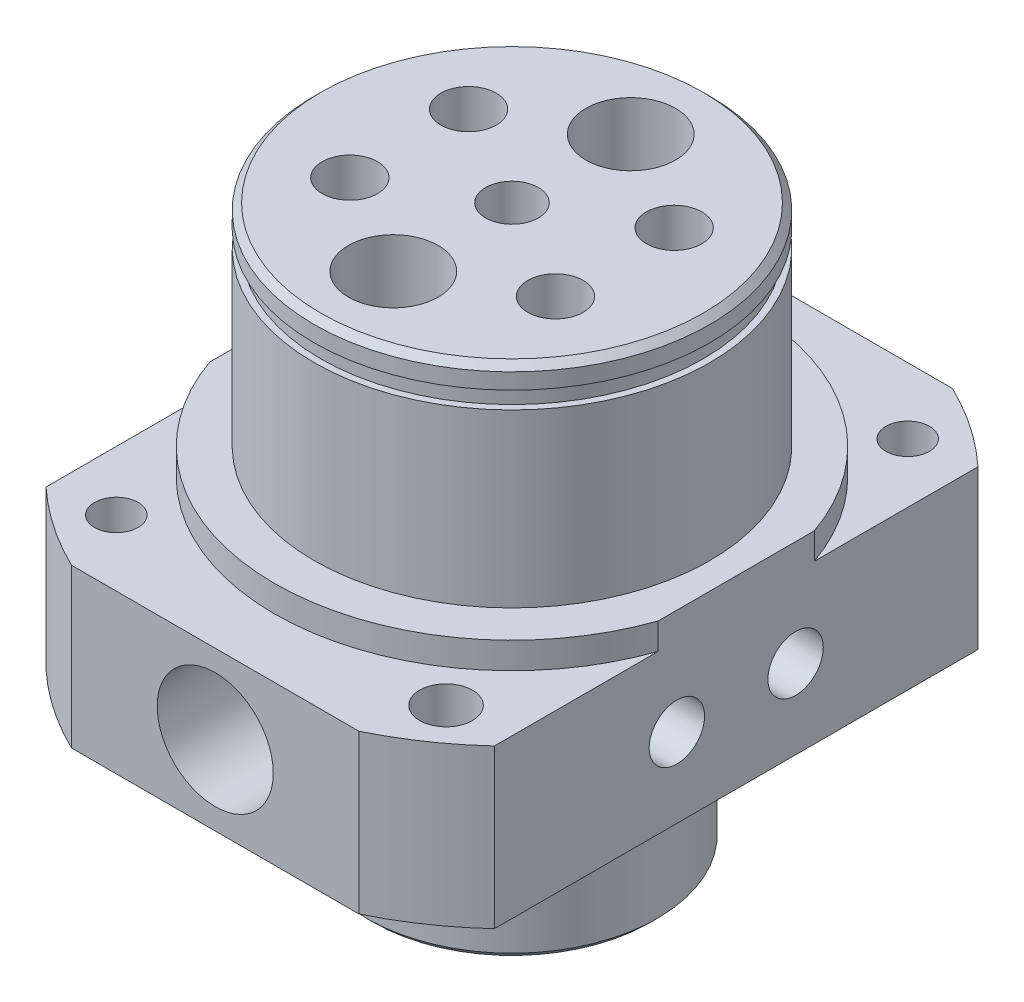
from build123d import *

# Parameters (mm, degrees)
SKETCH2_OUTSIDE_W        = 68.448
SKETCH2_OUTSIDE_H        = 68.448
SKETCH2_OUTSIDE_W_2      = 34
SKETCH2_OUTSIDE_H_2      = 45
CUT_EXTRUDE1_DEPTH       = 47.368092477
M4_TAPPED_HOLE1_D        = 3.3
SKETCH14_R               = 2
CUT_EXTRUDE5_DEPTH       = 38.030392923
SKETCH17_R               = 2
SKETCH17_R_2             = 3
CUT_EXTRUDE7_DEPTH       = 28
CUT_EXTRUDE10_REACH      = 52.619
SKETCH18_R               = 2
CUT_EXTRUDE11_REACH      = 52.619
SKETCH19_R               = 2
CUT_EXTRUDE12_REACH      = 58.692
CUT_EXTRUDE12_END_RADIUS = 3
SKETCH20_R               = 3
CUT_EXTRUDE13_REACH      = 58.692
CUT_EXTRUDE13_END_RADIUS = 3
SKETCH21_R               = 3
SKETCH22_R               = 2
CUT_EXTRUDE14_DEPTH      = 51.589030432
CHAMFER1_SIZE            = 0.5
M8_TAPPED_HOLE1_D        = 6.8
M8_TAPPED_HOLE1_DEPTH    = 15
M8_TAPPED_HOLE1_TIP      = 2.042926105
M5_TAPPED_HOLE2_D        = 4.2
M5_TAPPED_HOLE2_DEPTH    = 12
M5_TAPPED_HOLE2_TIP      = 1.2618073
M5_TAPPED_HOLE1_D        = 4.2
M5_TAPPED_HOLE1_DEPTH    = 12
M5_TAPPED_HOLE1_TIP      = 1.2618073
M5_TAPPED_HOLE3_D        = 4.2
M5_TAPPED_HOLE3_DEPTH    = 12
M5_TAPPED_HOLE3_TIP      = 1.2618073
G1_8_TAPPED_HOLE1_D      = 8.8
G1_8_TAPPED_HOLE1_DEPTH  = 15
G1_8_TAPPED_HOLE1_TIP    = 2.643786724
G1_8_TAPPED_HOLE2_D      = 8.8
G1_8_TAPPED_HOLE2_DEPTH  = 15
G1_8_TAPPED_HOLE2_TIP    = 2.643786724


with BuildPart() as part:
    # Sketch1 → Revolve1 (revolve)
    with BuildSketch(Plane(origin=(0, 0, 0), x_dir=(0, 0, -1), z_dir=(1, 0, 0)), mode=Mode.PRIVATE) as revolve1_sk:
        Polygon((0, -12), (11, -12), (11, 0), (25, 0), (25, 12), (18, 12), (18, 14), (15, 14), (15, 27), (14.5, 27), (14.5, 28.3), (15, 28.3), (15, 30), (0, 30), align=None)
    revolve(revolve1_sk.sketch.rotate(Axis((0, 78.762169225, 0), (0, -1, 0)), 180), axis=Axis((0, 78.762169225, 0), (0, -1, 0)))

    # Sketch2 outside → Cut-Extrude1 (cut, through all)
    with BuildSketch(Plane(origin=(0, 0, 0), x_dir=(1, 0, 0), z_dir=(0, 1, 0))):
        Rectangle(SKETCH2_OUTSIDE_W, SKETCH2_OUTSIDE_H)
        Rectangle(SKETCH2_OUTSIDE_W_2, SKETCH2_OUTSIDE_H_2, mode=Mode.SUBTRACT)
    extrude(amount=CUT_EXTRUDE1_DEPTH, mode=Mode.SUBTRACT)

    # M4 Tapped Hole1 (through all)
    with Locations(Plane(origin=(0, 0, 0), x_dir=(-1, 0, 0), z_dir=(0, -1, 0))):
        with Locations((-12.5, 17.5), (12.5, -17.5)):
            Hole(M4_TAPPED_HOLE1_D / 2)

    # Sketch14 → Cut-Extrude5 (cut, through all)
    with BuildSketch(Plane(origin=(0, 12, 0), x_dir=(1, 0, 0), z_dir=(0, 1, 0))):
        with Locations(Location((12.5, -17.5, 0), (0, 0, 270))):
            Circle(SKETCH14_R)
        with Locations(Location((-12.5, 17.5, 0), (0, 0, 270))):
            Circle(SKETCH14_R)
    extrude(amount=-CUT_EXTRUDE5_DEPTH, mode=Mode.SUBTRACT)

    # Sketch17 → Cut-Extrude7 (cut)
    with BuildSketch(Plane(origin=(0, 30, 0), x_dir=(1, 0, 0), z_dir=(0, 1, 0))):
        with Locations(Location((-7.794228634, 4.5, 0), (0, 0, 270))):
            Circle(SKETCH17_R)
        with Locations(Location((-7.794228634, -4.5, 0), (0, 0, 270))):
            Circle(SKETCH17_R)
        with Locations(Location((0, -9, 0), (0, 0, 270))):
            Circle(SKETCH17_R_2)
        with Locations(Location((7.794228634, 4.5, 0), (0, 0, 270))):
            Circle(SKETCH17_R)
        with Locations(Location((0, 9, 0), (0, 0, 270))):
            Circle(SKETCH17_R_2)
        with Locations(Location((7.794228634, -4.5, 0), (0, 0, 270))):
            Circle(SKETCH17_R)
        with Locations(Location((0, 0, 0), (0, 0, 270))):
            Circle(SKETCH17_R)
    extrude(amount=-CUT_EXTRUDE7_DEPTH, mode=Mode.SUBTRACT)

    # Sketch18 → Cut-Extrude10 (cut, up to next)
    with BuildSketch(Plane.ZY.offset(17), mode=Mode.PRIVATE) as cut_extrude10_sk1:
        with Locations((-4.5, 6)):
            Circle(SKETCH18_R)
    cut_extrude10_tool1 = extrude(cut_extrude10_sk1.sketch, amount=-CUT_EXTRUDE10_REACH, mode=Mode.PRIVATE) & part.part
    # Sketch18 → Cut-Extrude10 (cut, up to next)
    with BuildSketch(Plane.ZY.offset(17), mode=Mode.PRIVATE) as cut_extrude10_sk2:
        with Locations((4.5, 6)):
            Circle(SKETCH18_R)
    cut_extrude10_tool2 = extrude(cut_extrude10_sk2.sketch, amount=-CUT_EXTRUDE10_REACH, mode=Mode.PRIVATE) & part.part
    add(cut_extrude10_tool1.solids().sort_by_distance((-17, 6, -4.5))[0], mode=Mode.SUBTRACT)
    add(cut_extrude10_tool2.solids().sort_by_distance((-17, 6, 4.5))[0], mode=Mode.SUBTRACT)

    # Sketch19 → Cut-Extrude11 (cut, up to next)
    with BuildSketch(Plane(origin=(17, 0, 0), x_dir=(0, 0, -1), z_dir=(1, 0, 0)), mode=Mode.PRIVATE) as cut_extrude11_sk1:
        with Locations(Location((-4.5, 6, 0), (0, 0, 180))):
            Circle(SKETCH19_R)
    cut_extrude11_tool1 = extrude(cut_extrude11_sk1.sketch, amount=-CUT_EXTRUDE11_REACH, mode=Mode.PRIVATE) & part.part
    # Sketch19 → Cut-Extrude11 (cut, up to next)
    with BuildSketch(Plane(origin=(17, 0, 0), x_dir=(0, 0, -1), z_dir=(1, 0, 0)), mode=Mode.PRIVATE) as cut_extrude11_sk2:
        with Locations(Location((4.5, 6, 0), (0, 0, 180))):
            Circle(SKETCH19_R)
    cut_extrude11_tool2 = extrude(cut_extrude11_sk2.sketch, amount=-CUT_EXTRUDE11_REACH, mode=Mode.PRIVATE) & part.part
    add(cut_extrude11_tool1.solids().sort_by_distance((17, 6, 4.5))[0], mode=Mode.SUBTRACT)
    add(cut_extrude11_tool2.solids().sort_by_distance((17, 6, -4.5))[0], mode=Mode.SUBTRACT)

    # Cut-Extrude12: up to this cylinder (the profile starts outside it)
    cut_extrude12_end = Plane(origin=(0, 6, -9), z_dir=(0, 1, 0)) * Cylinder(CUT_EXTRUDE12_END_RADIUS, 124.384, mode=Mode.PRIVATE)
    # Sketch20 → Cut-Extrude12 (cut, up to the surface)
    with BuildSketch(Plane(origin=(0, 0, -22.5), x_dir=(-1, 0, 0), z_dir=(0, 0, -1)), mode=Mode.PRIVATE) as cut_extrude12_sk1:
        with Locations((0, 6)):
            Circle(SKETCH20_R)
    cut_extrude12_tool1 = extrude(cut_extrude12_sk1.sketch, amount=-CUT_EXTRUDE12_REACH, mode=Mode.PRIVATE) - cut_extrude12_end
    add(cut_extrude12_tool1.solids().sort_by_distance((0, 6, -22.5))[0], mode=Mode.SUBTRACT)

    # Cut-Extrude13: up to this cylinder (the profile starts outside it)
    cut_extrude13_end = Plane(origin=(0, 6, 9), z_dir=(0, 1, 0)) * Cylinder(CUT_EXTRUDE13_END_RADIUS, 124.384, mode=Mode.PRIVATE)
    # Sketch21 → Cut-Extrude13 (cut, up to the surface)
    with BuildSketch(Plane.XY.offset(22.5), mode=Mode.PRIVATE) as cut_extrude13_sk1:
        with Locations(Location((0, 6, 0), (0, 0, 180))):
            Circle(SKETCH21_R)
    cut_extrude13_tool1 = extrude(cut_extrude13_sk1.sketch, amount=-CUT_EXTRUDE13_REACH, mode=Mode.PRIVATE) - cut_extrude13_end
    add(cut_extrude13_tool1.solids().sort_by_distance((0, 6, 22.5))[0], mode=Mode.SUBTRACT)

    # Sketch22 → Cut-Extrude14 (cut, through all)
    with BuildSketch(Plane.XZ.offset(12)):
        with Locations(Location((0, 0, 0), (0, 0, 90))):
            Circle(SKETCH22_R)
    extrude(amount=-CUT_EXTRUDE14_DEPTH, mode=Mode.SUBTRACT)

    # Chamfer1
    chamfer1_edges = [part.edges().sort_by_distance(p)[0] for p in [
        (0, -12, -11),
        (0, 30, -15),
    ]]
    chamfer(chamfer1_edges, length=CHAMFER1_SIZE)

    # M8 Tapped Hole1
    with Locations(Plane(origin=(0, 30, 0), x_dir=(1, 0, 0), z_dir=(0, 1, 0))):
        with Locations((0, 9), (0, -9)):
            Hole(M8_TAPPED_HOLE1_D / 2, depth=M8_TAPPED_HOLE1_DEPTH)
            with Locations((0, 0, -(M8_TAPPED_HOLE1_DEPTH + M8_TAPPED_HOLE1_TIP / 2))):  # 118° drill point
                Cone(0, M8_TAPPED_HOLE1_D / 2, M8_TAPPED_HOLE1_TIP, mode=Mode.SUBTRACT)

    # M5 Tapped Hole2
    with Locations(Plane(origin=(0, 30, 0), x_dir=(1, 0, 0), z_dir=(0, 1, 0))):
        with Locations((7.794228634, 4.5), (7.794228634, -4.5), (-7.794228634, -4.5), (-7.794228634, 4.5)):
            Hole(M5_TAPPED_HOLE2_D / 2, depth=M5_TAPPED_HOLE2_DEPTH)
            with Locations((0, 0, -(M5_TAPPED_HOLE2_DEPTH + M5_TAPPED_HOLE2_TIP / 2))):  # 118° drill point
                Cone(0, M5_TAPPED_HOLE2_D / 2, M5_TAPPED_HOLE2_TIP, mode=Mode.SUBTRACT)

    # M5 Tapped Hole1
    with Locations(Plane.ZY.offset(17)):
        with Locations((-4.5, 6), (4.5, 6)):
            Hole(M5_TAPPED_HOLE1_D / 2, depth=M5_TAPPED_HOLE1_DEPTH)
            with Locations((0, 0, -(M5_TAPPED_HOLE1_DEPTH + M5_TAPPED_HOLE1_TIP / 2))):  # 118° drill point
                Cone(0, M5_TAPPED_HOLE1_D / 2, M5_TAPPED_HOLE1_TIP, mode=Mode.SUBTRACT)

    # M5 Tapped Hole3
    with Locations(Plane(origin=(17, 0, 0), x_dir=(0, 0, -1), z_dir=(1, 0, 0))):
        with Locations((4.5, 6), (-4.5, 6)):
            Hole(M5_TAPPED_HOLE3_D / 2, depth=M5_TAPPED_HOLE3_DEPTH)
            with Locations((0, 0, -(M5_TAPPED_HOLE3_DEPTH + M5_TAPPED_HOLE3_TIP / 2))):  # 118° drill point
                Cone(0, M5_TAPPED_HOLE3_D / 2, M5_TAPPED_HOLE3_TIP, mode=Mode.SUBTRACT)

    # G1/8 Tapped Hole1
    with Locations(Plane.XY.offset(22.5)):
        with Locations((0, 6)):
            Hole(G1_8_TAPPED_HOLE1_D / 2, depth=G1_8_TAPPED_HOLE1_DEPTH)
            with Locations((0, 0, -(G1_8_TAPPED_HOLE1_DEPTH + G1_8_TAPPED_HOLE1_TIP / 2))):  # 118° drill point
                Cone(0, G1_8_TAPPED_HOLE1_D / 2, G1_8_TAPPED_HOLE1_TIP, mode=Mode.SUBTRACT)

    # G1/8 Tapped Hole2
    with Locations(Plane(origin=(0, 0, -22.5), x_dir=(-1, 0, 0), z_dir=(0, 0, -1))):
        with Locations((0, 6)):
            Hole(G1_8_TAPPED_HOLE2_D / 2, depth=G1_8_TAPPED_HOLE2_DEPTH)
            with Locations((0, 0, -(G1_8_TAPPED_HOLE2_DEPTH + G1_8_TAPPED_HOLE2_TIP / 2))):  # 118° drill point
                Cone(0, G1_8_TAPPED_HOLE2_D / 2, G1_8_TAPPED_HOLE2_TIP, mode=Mode.SUBTRACT)


solid = part.part
